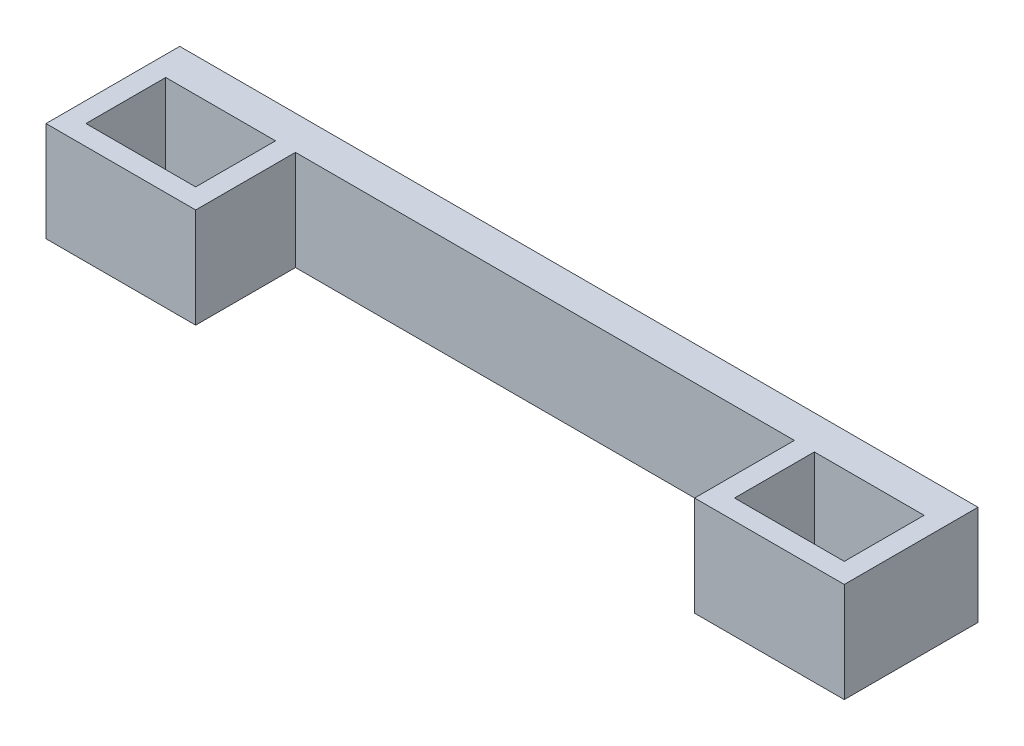
from build123d import *

# Parameters (mm, degrees)
SKETCH1_W           = 800
SKETCH1_H           = 134
BOSS_EXTRUDE1_DEPTH = 100
SKETCH2_W           = 500
SKETCH2_H           = 200
CUT_EXTRUDE1_DEPTH  = 100
SKETCH3_W           = 110
SKETCH3_H           = 80
CUT_EXTRUDE2_DEPTH  = 80


with BuildPart() as part:
    # Sketch1 → Boss-Extrude1 (new body)
    with BuildSketch(Plane(origin=(0, 0, 0), x_dir=(1, 0, 0), z_dir=(0, 1, 0))):
        Rectangle(SKETCH1_W, SKETCH1_H)
    extrude(amount=BOSS_EXTRUDE1_DEPTH)

    # Sketch2 → Cut-Extrude1 (cut)
    with BuildSketch(Plane(origin=(0, 100, 0), x_dir=(1, 0, 0), z_dir=(0, 1, 0))):
        with Locations((0, -67)):
            Rectangle(SKETCH2_W, SKETCH2_H)
    extrude(amount=-CUT_EXTRUDE1_DEPTH, mode=Mode.SUBTRACT)

    # Sketch3 → Cut-Extrude2 (cut)
    with BuildSketch(Plane(origin=(0, 100, 0), x_dir=(1, 0, 0), z_dir=(0, 1, 0))):
        with Locations((-325, -7)):
            Rectangle(SKETCH3_W, SKETCH3_H)
    cut_extrude2 = extrude(amount=-CUT_EXTRUDE2_DEPTH, mode=Mode.SUBTRACT)

    # Mirror1: Cut-Extrude2 across plane
    add(cut_extrude2.mirror(Plane(origin=(0, 0, 0), x_dir=(0, 0, 1), z_dir=(1, 0, 0))), mode=Mode.SUBTRACT)


solid = part.part
